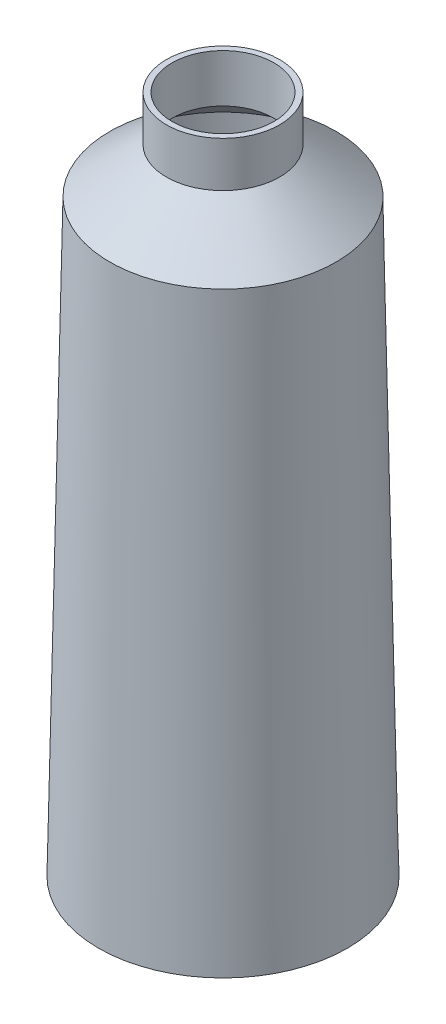
from build123d import *

# Parameters (mm, degrees)
SHELL1_T = -2.5


with BuildPart() as part:
    # Sketch1 → Revolve1 (revolve)
    with BuildSketch(Plane.XY, mode=Mode.PRIVATE) as revolve1_sk:
        Polygon((0, 0), (0, 300), (25, 300), (25, 280), (50, 260), (55, 0), align=None)
    revolve(revolve1_sk.sketch.rotate(Axis((0, 0, 0), (0, 1, 0)), 90), axis=Axis((0, 0, 0), (0, 1, 0)))

    # Shell1
    shell1_openings = [part.faces().sort_by_distance(p)[0] for p in [
        (0, 300, 0),
        (0, 0, 0),
    ]]
    offset(amount=SHELL1_T, openings=shell1_openings, kind=Kind.INTERSECTION)


solid = part.part
